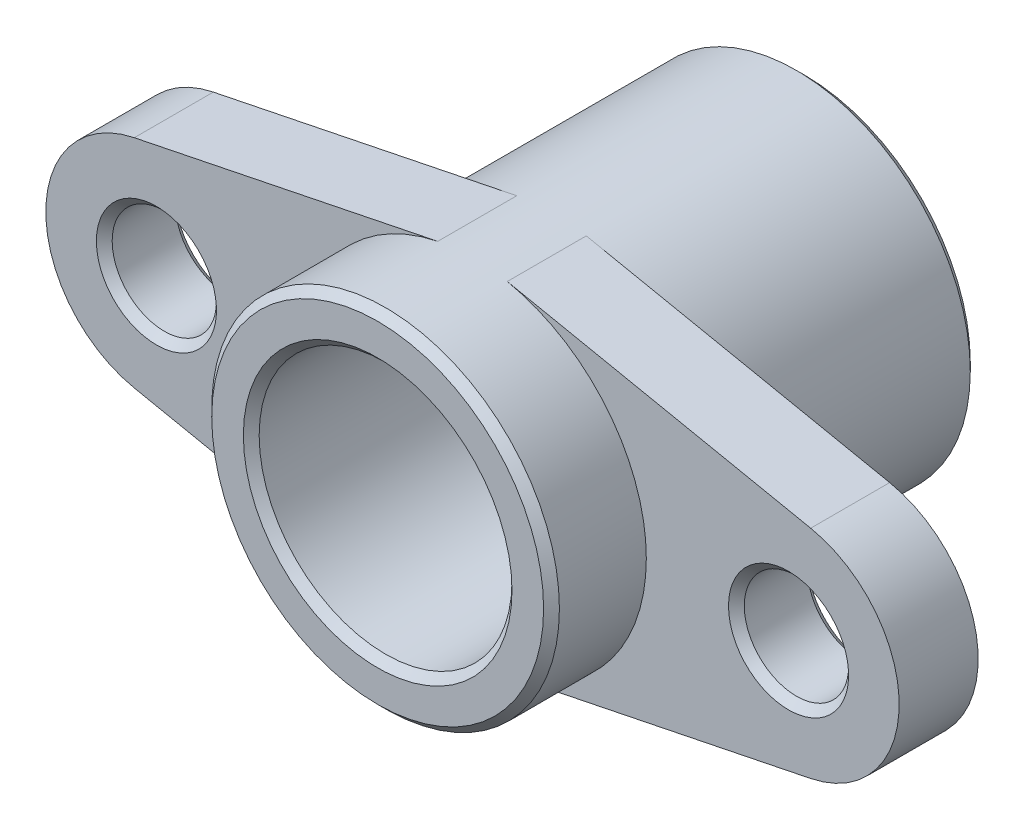
from build123d import *
from build123d.topology import SkipClean

# Parameters (mm, degrees)
SKETCH1_R                                            = 11
SKETCH1_R_2                                          = 8
BOSS_EXTRUDE1_DEPTH                                  = 30
BOSS_EXTRUDE2_START                                  = -14
SKETCH2_R                                            = 8
BOSS_EXTRUDE2_DEPTH                                  = 14
HOLE_SIZE_PER_SOCKET_HEAD_CAP_SCREW_TYPE_D           = 6.6
HOLE_SIZE_PER_SOCKET_HEAD_CAP_SCREW_TYPE_CBORE_D     = 15
HOLE_SIZE_PER_SOCKET_HEAD_CAP_SCREW_TYPE_CBORE_DEPTH = 9
SKETCH5_OUTSIDE_W                                    = 69.114
SKETCH5_OUTSIDE_H                                    = 37.114
SKETCH5_OUTSIDE_R                                    = 11
CUT_EXTRUDE2_DEPTH                                   = 9
CUT_EXTRUDE3_START                                   = -3
SKETCH6_R                                            = 11
CUT_EXTRUDE3_DEPTH                                   = 3
CHAMFER1_SIZE                                        = 0.5


with BuildPart() as part:
    # Sketch1 → Boss-Extrude1 (new body)
    with BuildSketch(Plane.XY):
        Circle(SKETCH1_R)
        Circle(SKETCH1_R_2, mode=Mode.SUBTRACT)
    extrude(amount=BOSS_EXTRUDE1_DEPTH)

    # Sketch2 → Boss-Extrude2 (add)
    with SkipClean():  # the faces are left unmerged after this step: merging them gives an invalid solid
        with BuildSketch(Plane.XY.offset(30).offset(BOSS_EXTRUDE2_START)):
            with BuildLine():
                Line((-21.4, 6.858571), (-2.2, 10.777755))
                ThreePointArc((-2.2, 10.777755), (0, 11), (2.2, 10.777755))
                Line((2.2, 10.777755), (21.4, 6.858571))
                ThreePointArc((21.4, 6.858571), (27, 0), (21.4, -6.858571))
                Line((21.4, -6.858571), (2.2, -10.777755))
                ThreePointArc((2.2, -10.777755), (0, -11), (-2.2, -10.777755))
                Line((-2.2, -10.777755), (-21.4, -6.858571))
                ThreePointArc((-21.4, -6.858571), (-27, 0), (-21.4, 6.858571))
            make_face()
            Circle(SKETCH2_R, mode=Mode.SUBTRACT)
        extrude(amount=BOSS_EXTRUDE2_DEPTH)

    # Hole size per socket head cap screw type1 (through all)
    with Locations(Plane(origin=(-20, 0, 30), x_dir=(1, 0, 0), z_dir=(0, 0, 1))):
        with Locations((0, 0), (40, 0)):
            CounterBoreHole(HOLE_SIZE_PER_SOCKET_HEAD_CAP_SCREW_TYPE_D / 2, HOLE_SIZE_PER_SOCKET_HEAD_CAP_SCREW_TYPE_CBORE_D / 2, HOLE_SIZE_PER_SOCKET_HEAD_CAP_SCREW_TYPE_CBORE_DEPTH)

    # Sketch5 outside → Cut-Extrude2 (cut)
    with SkipClean():  # the faces are left unmerged after this step: merging them gives an invalid solid
        with BuildSketch(Plane.XY.offset(30)):
            Rectangle(SKETCH5_OUTSIDE_W, SKETCH5_OUTSIDE_H)
            Circle(SKETCH5_OUTSIDE_R, mode=Mode.SUBTRACT)
        extrude(amount=-CUT_EXTRUDE2_DEPTH, mode=Mode.SUBTRACT)

    # Sketch6 → Cut-Extrude3 (cut)
    with SkipClean():  # the faces are left unmerged after this step: merging them gives an invalid solid
        with BuildSketch(Plane.XY.offset(30).offset(CUT_EXTRUDE3_START)):
            Circle(SKETCH6_R)
        extrude(amount=CUT_EXTRUDE3_DEPTH, mode=Mode.SUBTRACT)

    # Chamfer1
    chamfer1_edges = [part.edges().sort_by_distance(p)[0] for p in [
        (8.520563, 6.957011, 27),
        (-8, 0, 27),
        (-11, 0, 0),
        (23.3, 0, 16),
        (23.3, 0, 21),
        (-8, 0, 0),
        (-16.7, 0, 16),
        (-16.7, 0, 21),
    ]]
    chamfer(chamfer1_edges, length=CHAMFER1_SIZE)


solid = part.part
